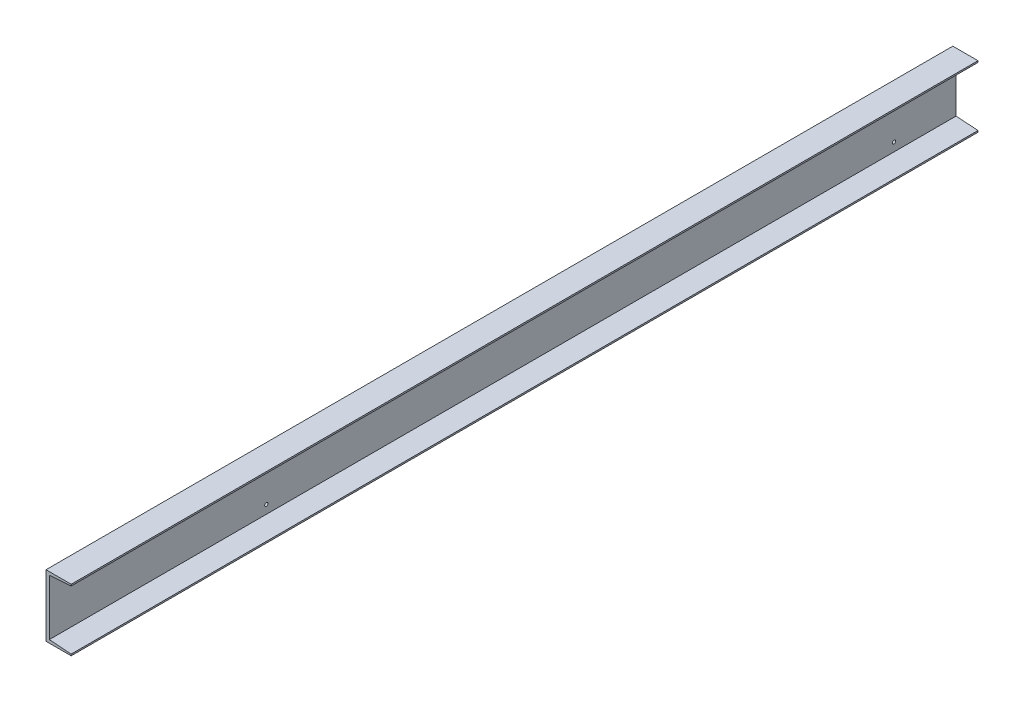
SolidWorks part; units mm, degrees
material "A3"
ref_plane "前视基准面" through (0, 0, 0) normal (0, 0, 1) x (1, 0, 0)
ref_plane "上视基准面" through (0, 0, 0) normal (0, 1, 0) x (1, 0, 0)
ref_plane "右视基准面" through (0, 0, 0) normal (1, 0, 0) x (0, 0, -1)
sketch "草图1" plane through (0, 0, 0) normal (0, 0, 1) x (1, 0, 0)
  line L0 (0, 0) -> (65, 0)
  line L1 (0, 0) -> (0, 160)
  line L2 (65, 156) -> (8.5, 152)
  line L3 (65, 0) -> (65, 4)
  line L4 (65, 4) -> (8.5, 8)
  line L5 (8.5, 8) -> (8.5, 152)
  line L6 (0, 80) -> (8.5, 80) construction
  line L7 (65, 160) -> (65, 156)
  line L8 (0, 160) -> (65, 160)
  dimension "D1" = 160
  dimension "D2" = 65
  dimension "D3" = 4
  dimension "D4" = 8.5
  dimension "D5" = 144
extrude "凸台-拉伸1" add sketch "草图1" along normal mid plane 2340
hole_wizard "M10 螺纹孔1" positions "草图2" profile "草图3" tap size "M10" standard "GB"
sketch "草图2" plane through (0, 0, 0) normal (-1, 0, 0) x (0, 0, 1)
  line L3 (-1170, 160) -> (-1170, 0) construction
  line L4 (-1170, 80) -> (1170, 80) construction
  line L5 (1170, 160) -> (1170, 0) construction
  point P0 (-1010, 30)
  point P11 (610, 30)
  point P17 (-1010, 130)
  point P18 (610, 130)
  point P23 (-1170, 80)
  point P36 (610, 130)
  point P37 (-1010, 130)
  dimension "D1" = 100
  dimension "D2" = 160
  dimension "D5" = 560
  dimension "D3" = 2
  dimension "D4" = 2
sketch "草图3" plane through (0, 30, -1010) normal (0, 1, 0) x (0, 0, 1)
  line L0 (0, 0) -> (0, 30.0537)
  line L1 (0, 30.0537) -> (4.25, 27.5)
  line L2 (4.25, 27.5) -> (4.25, 0)
  line L5 (4.25, 0) -> (0, 0)
  line L10 (0, 30.0537) -> (-4.25, 27.5) construction
  line L11 (0, -6.35) -> (0, 107.95) construction
  dimension "螺纹孔钻头直径" = 8.5
  dimension "螺纹孔钻头深度" = 27.5
  dimension "导头角度" = 118
cosmetic thread "孔螺蚊线1" parameters "D1"=20, "D2"=10
cosmetic thread "孔螺蚊线4" parameters "D1"=20, "D2"=10
cosmetic thread "孔螺蚊线5" parameters "D1"=20, "D2"=10
cosmetic thread "孔螺蚊线6" parameters "D1"=20, "D2"=10
